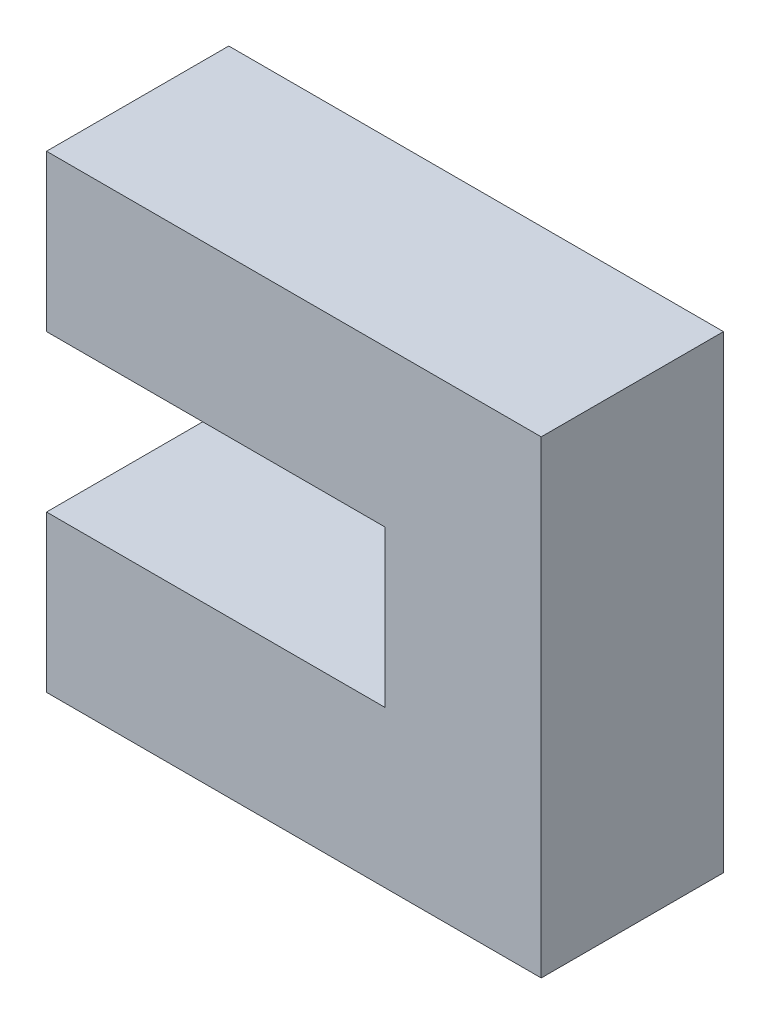
from build123d import *

# Parameters (mm, degrees)
EXTRUDE_1_DEPTH = 3.5


with BuildPart() as part:
    # 草图1 → 凸台-拉伸1 (new, symmetric)
    with BuildSketch(Plane.XY):
        Polygon((0, 0), (0, 9), (-19, 9), (-19, 3), (-6, 3), (-6, -3), (-19, -3), (-19, -9), (0, -9), align=None)
    extrude(amount=EXTRUDE_1_DEPTH, both=True)


solid = part.part
